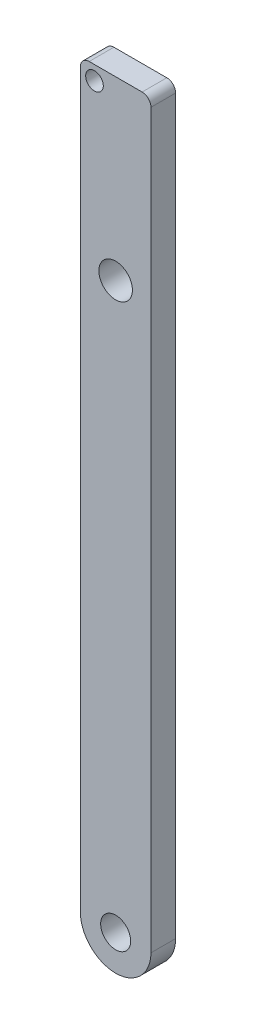
SolidWorks part; units mm, degrees
ref_plane "前视基准面" through (0, 0, 0) normal (0, 0, 1) x (1, 0, 0)
ref_plane "上视基准面" through (0, 0, 0) normal (0, 1, 0) x (1, 0, 0)
ref_plane "右视基准面" through (0, 0, 0) normal (1, 0, 0) x (0, 0, -1)
sketch "草图1" plane through (0, 0, 0) normal (0, 0, 1) x (1, 0, 0)
  line L1 (-15, 220) -> (15, 220)
  line L2 (-20, 215) -> (-20, -200)
  line L4 (20, 215) -> (20, -200)
  arc A0 (-20, -200) -> (20, -200) centre (0, -200) ccw
  arc A1 (15, 220) -> (20, 215) centre (15, 215) cw
  arc A2 (-15, 220) -> (-20, 215) centre (-15, 215) ccw
  circle A3 centre (0, 120) radius 9.5
  circle A4 centre (0, -200) radius 8.5
  point P0 (0, 0)
  point P8 (20, 220)
  point P12 (-20, 220)
  dimension "D2" = 5
  dimension "D5" = 200
  dimension "D7" = 19
  dimension "D8" = 17
  dimension "D1" = 40
  dimension "D3" = 415
  dimension "D4" = 220
  dimension "D6" = 100
  dimension "D9" = 20
extrude "凸台-拉伸1" add sketch "草图1" along normal blind 14
sketch "草图2" plane through (0, 0, 0) normal (0, 0, -1) x (-1, 0, 0)
  line L0 (20, 215) -> (20, -200) construction
  line L1 (-15, 220) -> (15, 220) construction
  circle A0 centre (12, 212) radius 5
  dimension "D1" = 10
  dimension "D2" = 8
  dimension "D3" = 8
extrude "切除-拉伸1" cut sketch "草图2" against normal blind 20
